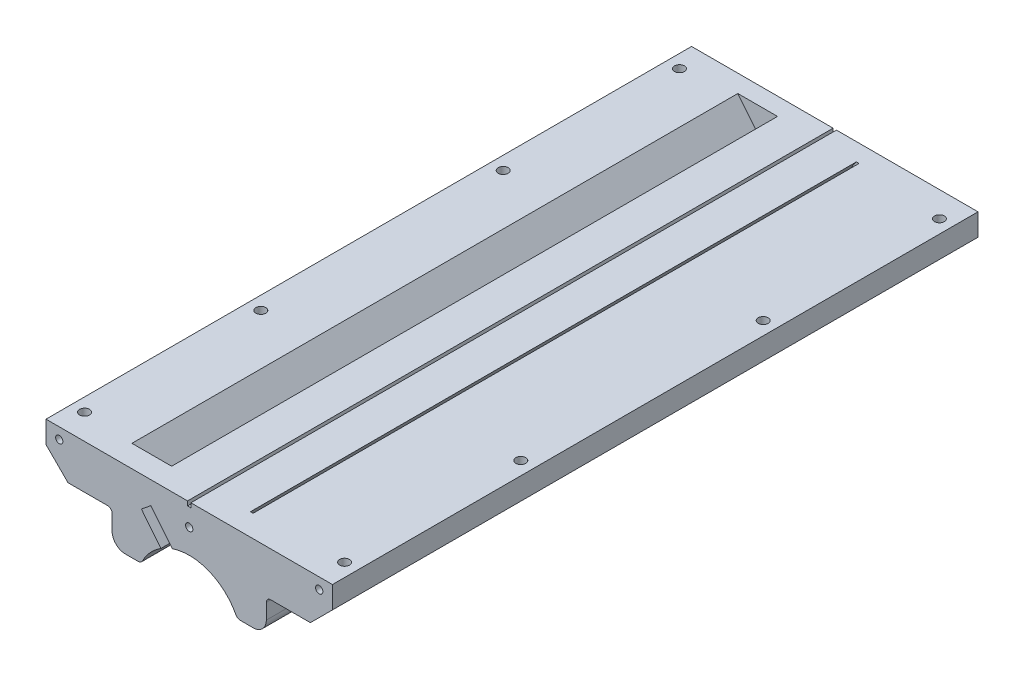
SolidWorks part; units mm, degrees
ref_plane "Front Plane" through (0, 0, 0) normal (0, 0, 1) x (1, 0, 0)
ref_plane "Top Plane" through (0, 0, 0) normal (0, 1, 0) x (1, 0, 0)
ref_plane "Right Plane" through (0, 0, 0) normal (1, 0, 0) x (0, 0, -1)
sketch "Sketch1" plane through (0, 0, 0) normal (0, 0, 1) x (1, 0, 0)
  line L1 (-65, 17.5) -> (65, 17.5)
  line L2 (-65, 17.5) -> (-65, -17.5)
  line L3 (-65, -17.5) -> (65, -17.5)
  line L4 (65, 17.5) -> (65, -17.5)
  line L5 (-65, 17.5) -> (65, -17.5) construction
  line L6 (-65, -17.5) -> (65, 17.5) construction
  point P0 (0, 0)
  dimension "D1" = 130
  dimension "D2" = 35
extrude "Boss-Extrude1" add sketch "Sketch1" along normal mid plane 293
sketch "Sketch3" plane through (0, 0, 146.5) normal (0, 0, 1) x (1, 0, 0)
  line L0 (-65, -17.5) -> (65, -17.5) construction
  circle A0 centre (0, -27.5) radius 24
  dimension "D1" = 48
  dimension "D2" = 10
extrude "Cut-Extrude2" cut sketch "Sketch3" against normal through all
sketch "Sketch7" plane through (0, -17.5, 0) normal (0, -1, 0) x (1, 0, 0)
  line L0 (-65, -146.5) -> (-21.8174, -146.5) construction
  line L1 (-65, 146.5) -> (-35, 146.5)
  line L2 (-65, 146.5) -> (-65, -146.5)
  line L3 (-65, -146.5) -> (-35, -146.5)
  line L4 (-35, 146.5) -> (-35, -146.5)
  line L5 (21.8174, -146.5) -> (65, -146.5) construction
  line L6 (65, 146.5) -> (35, 146.5)
  line L7 (65, 146.5) -> (65, -146.5)
  line L8 (65, -146.5) -> (35, -146.5)
  line L9 (35, 146.5) -> (35, -146.5)
  dimension "D1" = 70
extrude "Cut-Extrude5" cut sketch "Sketch7" against normal blind 15
fillet "Fillet1" radius 6 2 edges at (35, -17.5, 0) (-35, -17.5, 0)
chamfer "Chamfer1" distance 10 2 edges at (65, -2.5, 0) (-65, -2.5, 0)
fillet "Fillet2" radius 2 2 edges at (35, -2.5, 0) (-35, -2.5, 0)
ref_plane "Plane4" through (0, 0, 136.5) normal (0, 0, 1) x (1, 0, 0)
sketch "Sketch8" plane through (0, 0, 136.5) normal (0, 0, 1) x (1, 0, 0)
  line L0 (-36, 17.5) -> (-25.12, 26.3105)
  line L1 (-36, 17.5) -> (-11.1703, -13.1621)
  line L2 (-25.12, 26.3105) -> (-0.2902, -4.3517)
  line L3 (-11.1703, -13.1621) -> (-0.2902, -4.3517)
  line L4 (18.1808, 18.0736) -> (19, 17.5)
  line L5 (18.1808, 18.0736) -> (3.005, -3.5998)
  line L6 (19, 17.5) -> (3.8241, -4.1734)
  line L7 (3.005, -3.5998) -> (3.8241, -4.1734)
  line L8 (0, 0) -> (0, -41.3441) construction
  line L9 (65, 17.5) -> (-65, 17.5) construction
  line L10 (21.8174, -17.5) -> (29, -17.5) construction
  line L11 (-29, -17.5) -> (-21.8174, -17.5) construction
  line L12 (1.4576, -7.5532) -> (0, -27.5) construction
  line L13 (3.005, -3.5998) -> (0.2727, -7.5019) construction
  line L14 (3.8241, -4.1734) -> (1.4576, -7.5532) construction
  line L15 (0.2727, -7.5019) -> (0, -27.5) construction
  line L16 (0.2727, -7.5019) -> (-3.2568, -2.1566) construction
  line L17 (1.4576, -7.5532) -> (-1.5646, -2.9763) construction
  line L18 (0.322, -3.8919) -> (-2.1331, -3.8584) construction
  line L19 (0.322, -3.8919) -> (2.777, -3.9254) construction
  line L20 (0.322, -3.8919) -> (0.2727, -7.5019) construction
  arc A1 (21.8174, -17.5) -> (-21.8174, -17.5) centre (0, -27.5) ccw construction
  arc A3 (21.8174, -17.5) -> (-21.8174, -17.5) centre (0, -27.5) ccw construction
  circle A4 centre (0, -27.5) radius 20 construction
  dimension "D5" = 40
  dimension "D1" = 14
  dimension "D2" = 1
  dimension "D3" = 55
  dimension "D4" = 51
  dimension "D6" = 36
  dimension "D7" = 19
extrude "Cut-Extrude6" cut sketch "Sketch8" against normal offset from surface (275 mm away) 8 up to face at (0, -3.1036, -146.5)
sketch "Sketch10" plane through (0, 0, 146.5) normal (0, 0, 1) x (1, 0, 0)
  line L0 (-21.7054, 3.8202) -> (-17.4311, 7.2814)
  line L1 (-21.7054, 3.8202) -> (-9.119, -11.7227)
  line L2 (-17.4311, 7.2814) -> (-4.8447, -8.2615)
  line L3 (-9.119, -11.7227) -> (-4.8447, -8.2615)
  line L4 (-25.4181, 4.4325) -> (-14.5381, 13.243) construction
  line L5 (-36, 17.5) -> (-14.8362, -8.6351) construction
  line L6 (-0.9642, -3.5194) -> (-17.9854, 17.5) construction
  line L7 (-21.3381, 7.7364) -> (-19.5682, 5.5508) construction
  line L8 (-0.9642, -3.5194) -> (-17.9854, 17.5) construction
  arc A0 (21.8174, -17.5) -> (-21.8174, -17.5) centre (0, -27.5) ccw construction
  dimension "D2" = 38
  dimension "D4" = 6
  dimension "D1" = 5.5
  dimension "D3" = 20
extrude "Cut-Extrude8" cut sketch "Sketch10" against normal through all
fillet "Fillet3" radius 2 2 edges at (-21.8174, -17.5, 0) (21.8174, -17.5, 0)
hole_wizard "M4 Tapped Hole1" positions "Sketch12" profile "Sketch11" tap size "M4" standard "Gb"
sketch "Sketch12" plane through (0, 0, 146.5) normal (0, 0, 1) x (1, 0, 0)
  line L0 (65, 17.5) -> (-65, 17.5) construction
  point P0 (0, 7.5)
  point P2 (59, 12.5)
  point P5 (-59, 12.5)
  dimension "D1" = 10
sketch "Sketch11" plane through (0, 7.5, 146.5) normal (1, 0, 0) x (0, -1, 0)
  line L0 (0, 0) -> (0, 12.4914)
  line L1 (0, 12.4914) -> (1.65, 11.5)
  line L2 (1.65, 11.5) -> (1.65, 0)
  line L5 (1.65, 0) -> (0, 0)
  line L10 (0, 12.4914) -> (-1.65, 11.5) construction
  line L11 (0, -6.35) -> (0, 107.95) construction
  dimension "螺纹孔钻头直径" = 3.3
  dimension "螺纹孔钻头深度" = 11.5
  dimension "导头角度" = 118
cosmetic thread "Cosmetic thread 1" parameters "D1"=8, "D2"=4
cosmetic thread "Cosmetic thread 2" parameters "D1"=8, "D2"=4
cosmetic thread "Cosmetic thread 3" parameters "D1"=8, "D2"=4
mirror "Mirror1" about plane through (0, 0, 0) normal (0, 0, 1) of "M4 Tapped Hole1"
sketch "Sketch15" plane through (0, 0, -146.5) normal (0, 0, -1) x (-1, 0, 0)
  line L0 (-65, 17.5) -> (65, 17.5) construction
  line L1 (-0.75, 19.5) -> (0.75, 19.5)
  line L2 (-0.75, 19.5) -> (-0.75, 15.5)
  line L3 (-0.75, 15.5) -> (0.75, 15.5)
  line L4 (0.75, 19.5) -> (0.75, 15.5)
  line L5 (-0.75, 19.5) -> (0.75, 15.5) construction
  line L6 (-0.75, 15.5) -> (0.75, 19.5) construction
  point P0 (0, 17.5)
  dimension "D1" = 1.5
  dimension "D2" = 2
extrude "Cut-Extrude9" cut sketch "Sketch15" against normal through all
hole_wizard "Hole size per socket head cap screw type 1" positions "Sketch17" profile "Sketch16" counterbore size "M4" standard "Gb" end condition through all
sketch "Sketch17" plane through (0, -2.5, 0) normal (0, -1, 0) x (-1, 0, 0)
  line L0 (65, 146.5) -> (65, -146.5) construction
  line L1 (-65, -146.5) -> (-65, 146.5) construction
  line L2 (37, -146.5) -> (55, -146.5) construction
  point P0 (59, -135)
  point P2 (-59, -135)
  dimension "D1" = 6
  dimension "D2" = 6
  dimension "D3" = 11.5
sketch "Sketch16" plane through (-59, -2.5, 135) normal (1, 0, 0) x (0, 0, -1)
  line L0 (0, 0) -> (0, 20)
  line L1 (0, 20) -> (2.25, 20)
  line L3 (2.25, 20) -> (2.25, 15)
  line L4 (2.25, 15) -> (4, 15)
  line L5 (4, 15) -> (4, 0)
  line L7 (4, 0) -> (0, 0)
  line L11 (0, -6.35) -> (0, 107.95) construction
  dimension "通孔孔直径" = 4.5
  dimension "通孔孔深度" = 20
  dimension "柱形沉头孔直径" = 8
  dimension "柱形沉头孔深度" = 15
pattern_linear "LPattern1" count 2 spacing 80 along (0, 0, -1) of "Hole size per socket head cap screw type 1"
mirror "Mirror2" about plane through (0, 0, 0) normal (0, 0, 1) of "Hole size per socket head cap screw type 1", "LPattern1"
